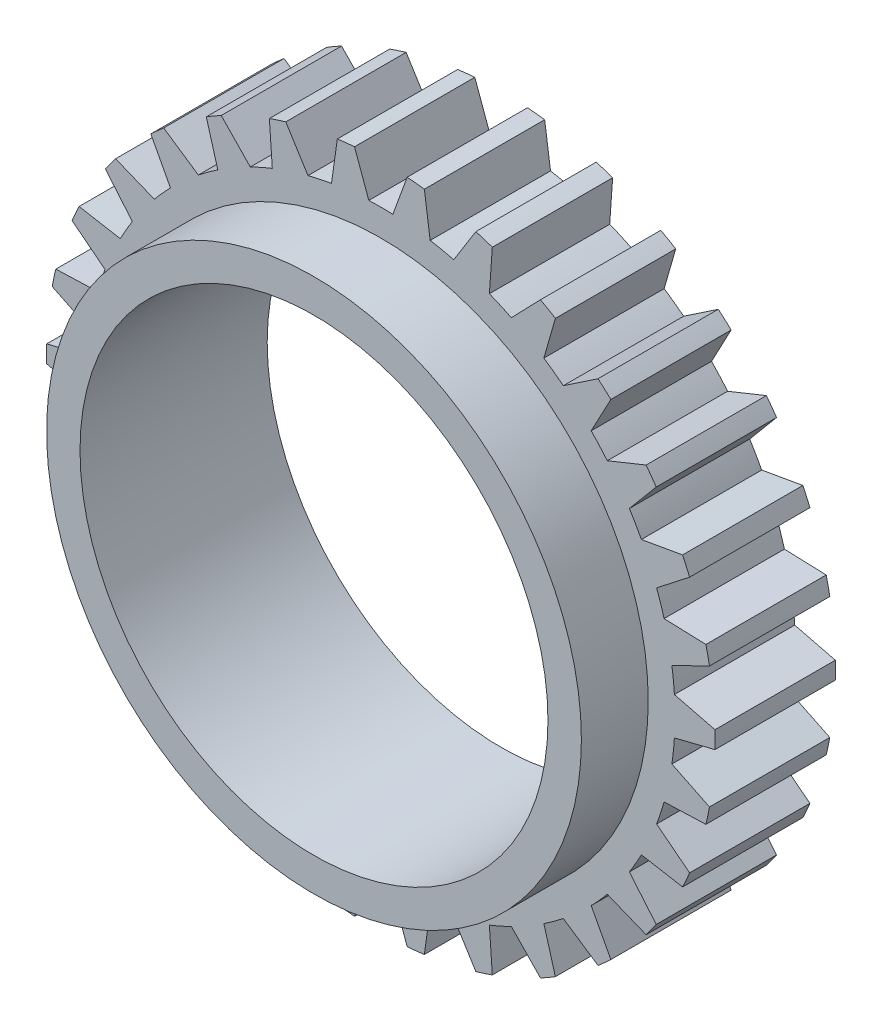
SolidWorks part; units mm, degrees
ref_plane "Front Plane" through (0, 0, 0) normal (0, 0, 1) x (1, 0, 0)
ref_plane "Top Plane" through (0, 0, 0) normal (0, 1, 0) x (1, 0, 0)
ref_plane "Right Plane" through (0, 0, 0) normal (1, 0, 0) x (0, 0, -1)
other "Configuration Table"
sketch "Sketch1" plane through (0, 0, 0) normal (1, 0, 0) x (0, 0, -1)
  line L0 (-22.6006, 0) -> (17.5251, 0) construction
  line L1 (0, 17.5) -> (0, 20)
  line L2 (0, 20) -> (5, 20)
  line L3 (5, 20) -> (5, 25)
  line L4 (5, 25) -> (14, 25)
  line L5 (14, 25) -> (14, 17.5)
  line L6 (14, 17.5) -> (0, 17.5)
  dimension "D1" = 35
  dimension "D2" = 40
  dimension "D3" = 50
  dimension "D4" = 14
  dimension "D5" = 9
revolve "Revolve1" add sketch "Sketch1" angle 360 about L0
cosmetic thread "Cosmetic Thread1" parameters "D2"=36
sketch "Sketch2" plane through (0, 0, -5) normal (0, 0, 1) x (1, 0, 0)
  line L0 (0, 27.5207) -> (0, -26.7364) construction
  line L1 (-0.9, -21.9816) -> (-1.9703, -24.9222)
  line L2 (0.9, -21.9816) -> (1.9703, -24.9222)
  circle A0 centre (0, 0) radius 22
  circle A1 centre (0, 0) radius 25
  circle M7 centre (0, 0) radius 25
  dimension "D1" = 50
  dimension "D2" = 44
  dimension "D3" = 1.8
  dimension "D4" = 40
extrude "Cut-Extrude1" cut sketch "Sketch2" against normal blind 10 contours L0 A0 L1 M7 | A0 L0 A1 L2
pattern_circular "CirPattern1" count 30 over 360 about axis through (0, 0, 0) along (0, 0, 1) of "Cut-Extrude1"
